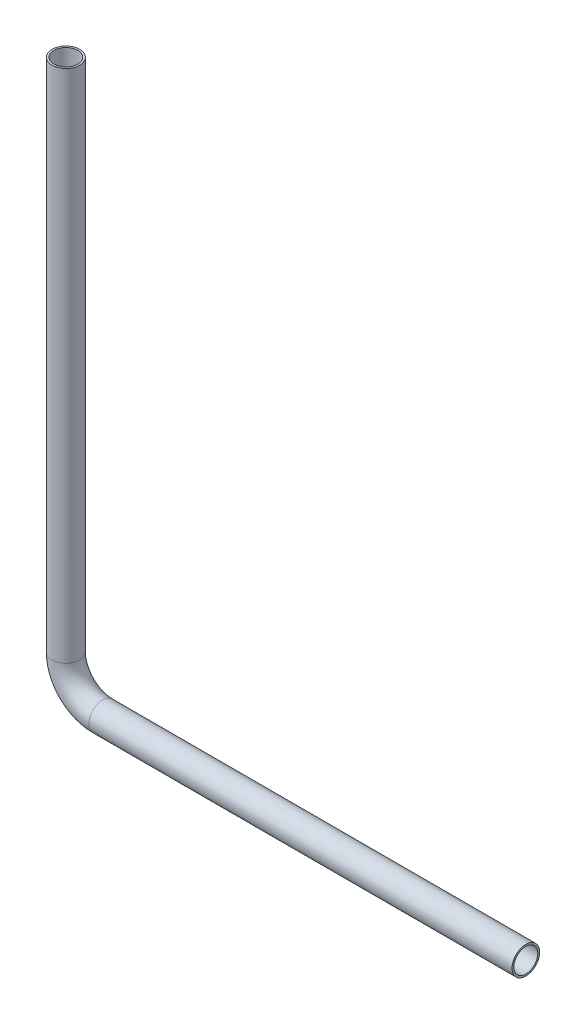
from build123d import *

# Parameters (mm, degrees)
SWEEP_THIN1_PROFILE_R   = 15
SWEEP_THIN1_PROFILE_R_2 = 13


with BuildPart() as part:
    # Sweep-Thin1: sweep along a path in Sketch1
    with BuildLine(Plane.XY) as sweep_thin1_path:
        Line((500, 0), (40, 0))
        ThreePointArc((40, 0), (11.715728753, 11.715728753), (0, 40))
        Line((0, 40), (0, 600))
    # Sweep-Thin1 profile (on start of the path) → Sweep-Thin1 (sweep)
    with BuildSketch(Plane(origin=(500, 0, 0), x_dir=(0, 0, -1), z_dir=(-1, 0, 0))):
        Circle(SWEEP_THIN1_PROFILE_R)
        Circle(SWEEP_THIN1_PROFILE_R_2, mode=Mode.SUBTRACT)
    sweep(path=sweep_thin1_path.line)


solid = part.part
